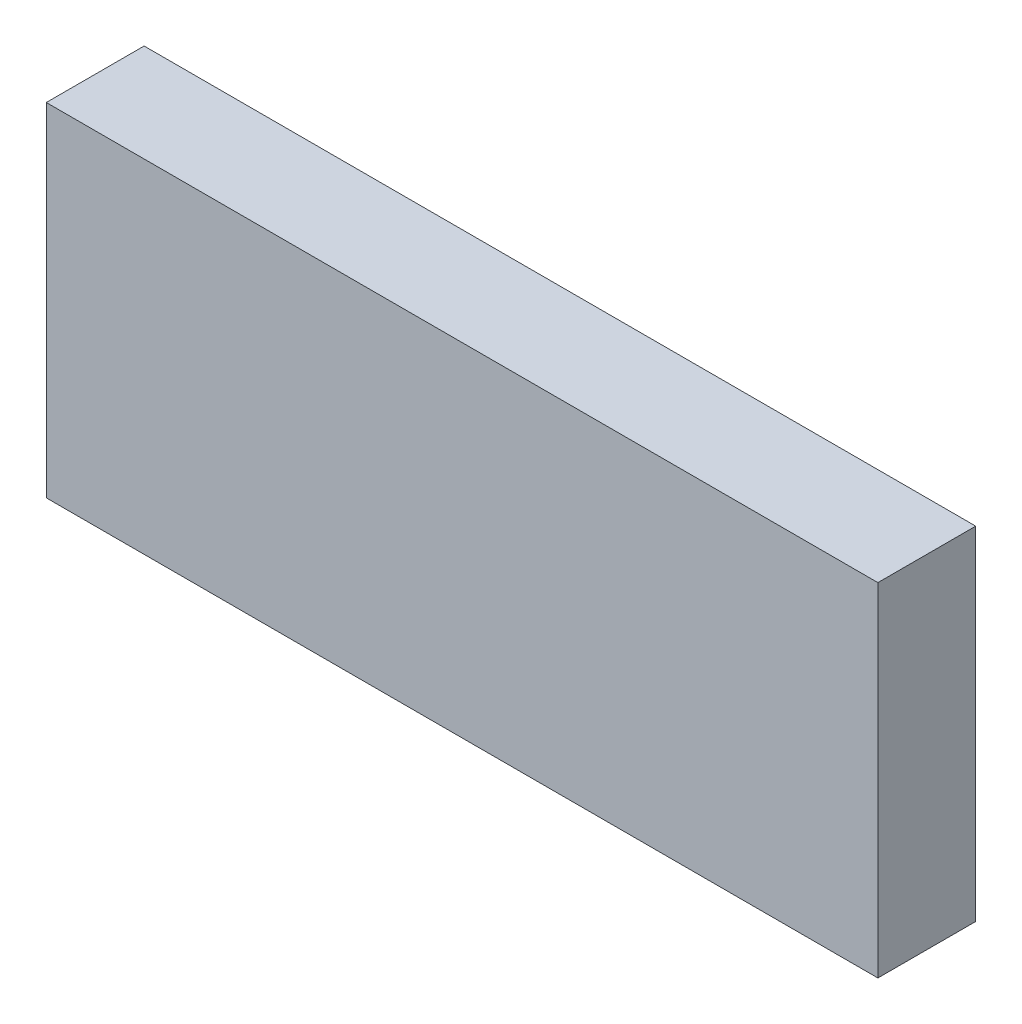
from build123d import *

# Parameters (mm, degrees)
SKETCH_1_W      = 170
SKETCH_1_H      = 70
EXTRUDE_1_DEPTH = 20


with BuildPart() as part:
    # 草图1 → 凸台-拉伸1 (new body)
    with BuildSketch(Plane.XY):
        Rectangle(SKETCH_1_W, SKETCH_1_H)
    extrude(amount=EXTRUDE_1_DEPTH)


solid = part.part
